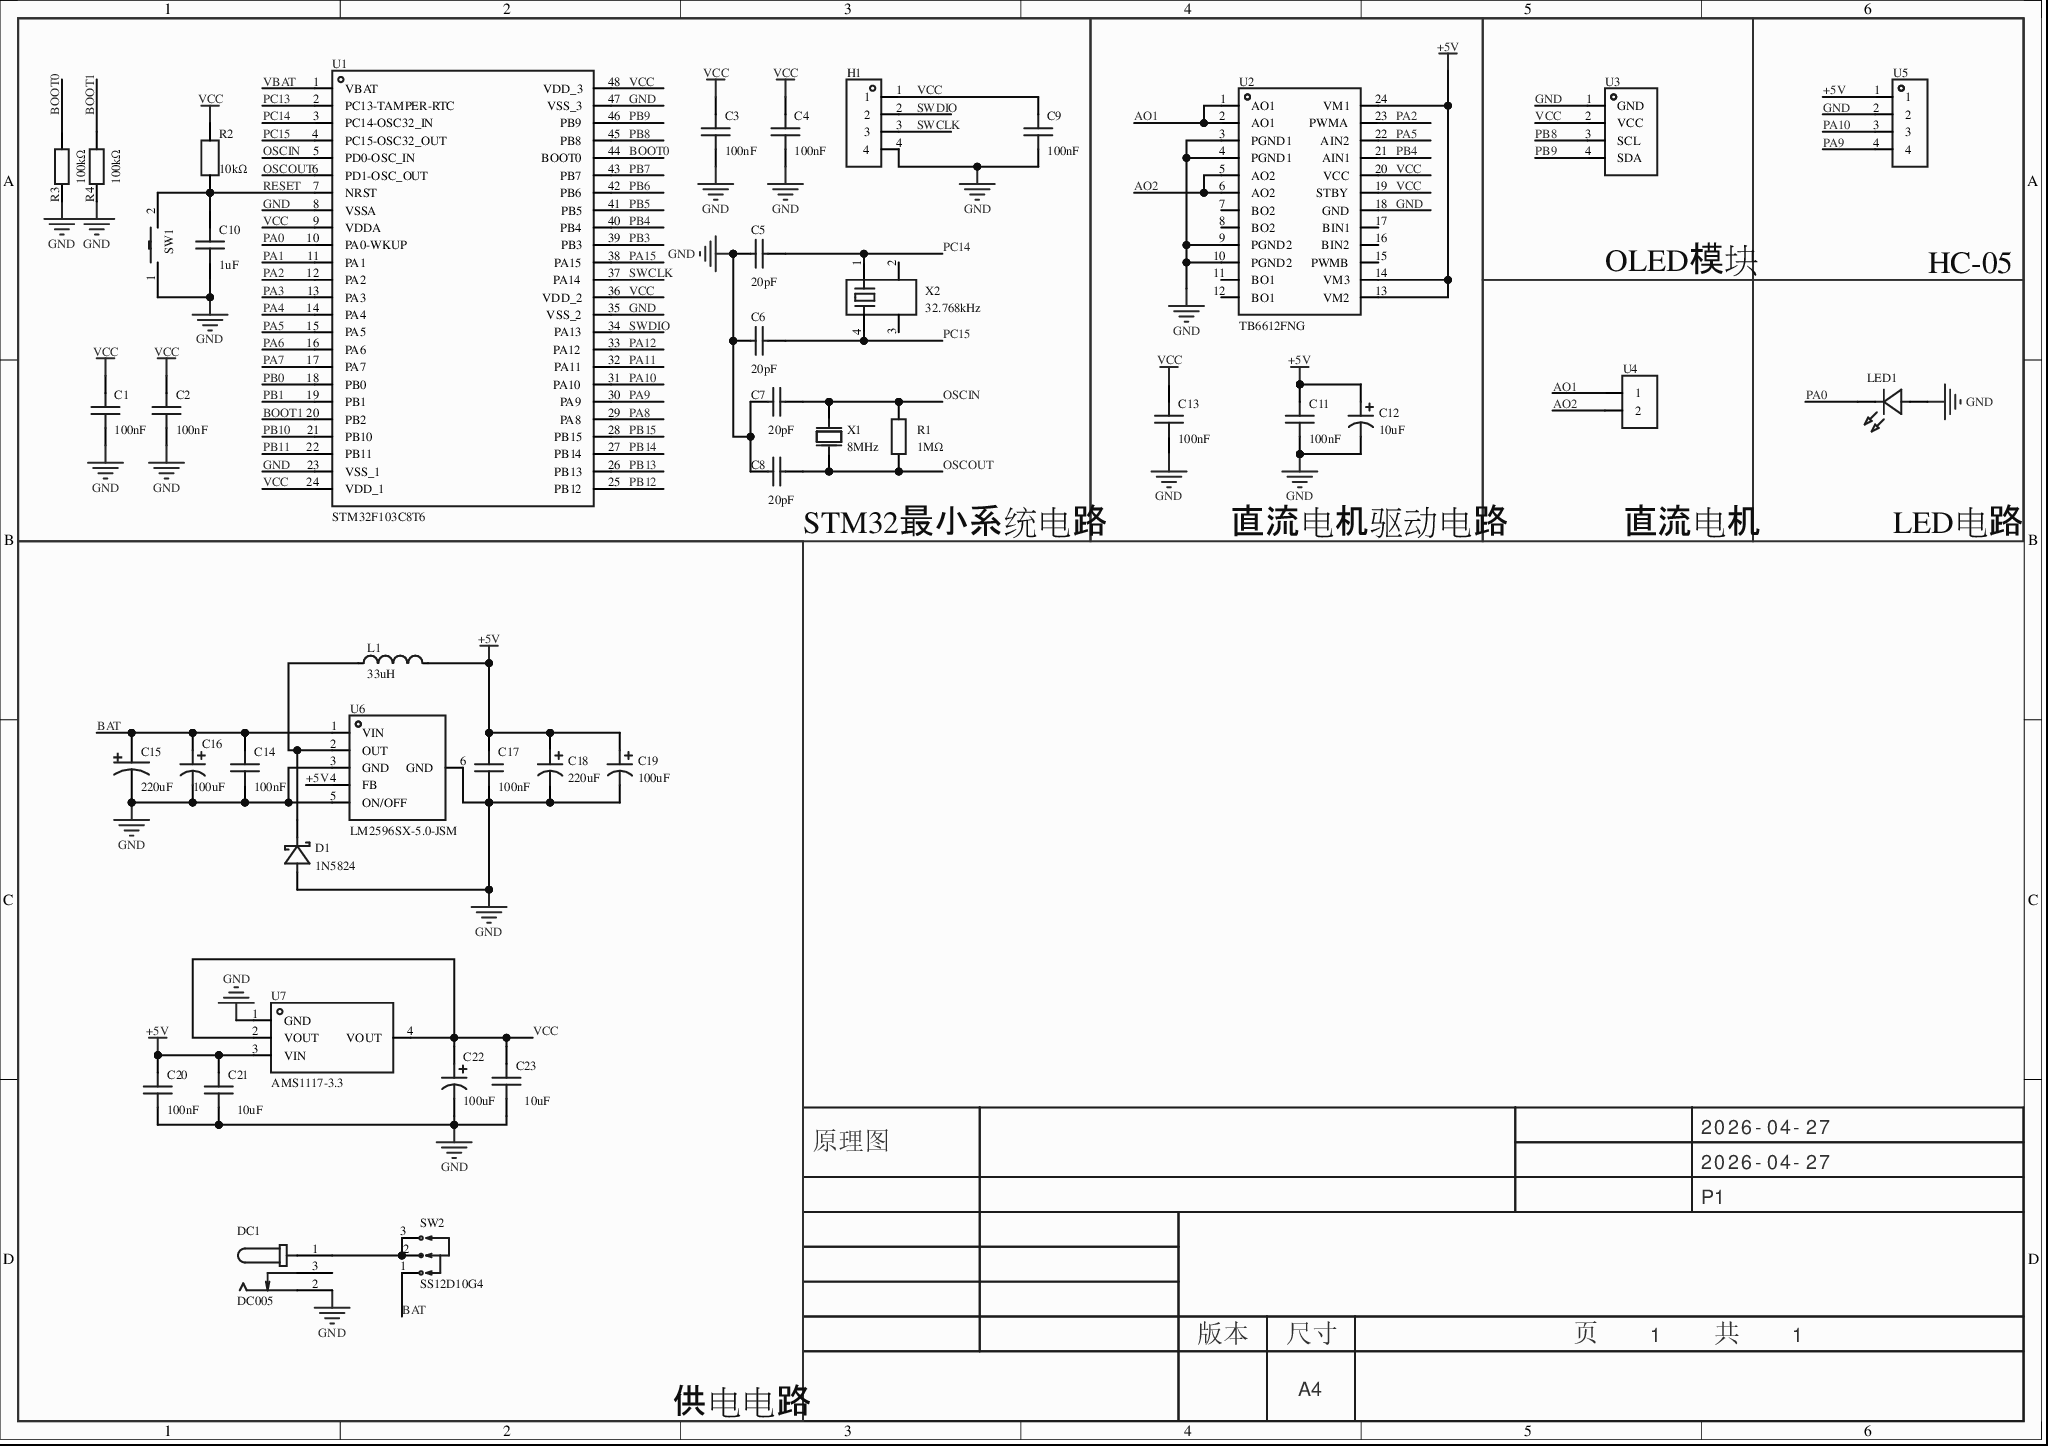
[diagram p0: MISC51997-3.schdoc]
# Altium project MISC51997-2.PrjPcb
1 sheet, 43 parts. Net scope: global (net labels, ports and power ports of the same name join across sheets).
Board file: MISC51997.pcbdoc

## Sheet MISC51997-3.schdoc
size 297 x 209 mm; Version: V1.0; @Project Name: MISC51997; @Update Date: 2026-04-27; @Create Date: 2026-04-27; @Board Name: MISC51997; @Create Time: 21:08:27; @Page Count: 1; @Page No: 1; @Schematic Name: MISC51997; @Update Time: 21:08:27; Size: A4

### Parts
C1  100nF  [C0603]
C2  100nF  [C0603]
C3  100nF  [C0603]
C4  100nF  [C0603]
C5  20pF  [C0603]
C6  20pF  [C0603]
C7  20pF  [C0603]
C8  20pF  [C0603]
C9  100nF  [C0603]
C10  1uF  [C0603]
C11  100nF  [C0603]
C12  10uF  [CAP-TH_BD5.0-P2.00-D0.5-FD-A]
C13  100nF  [C0603]
C14  100nF  [C0603]
C15  220uF  [CAP-TH_BD10.0-P5.00-D1.0-FD]
C16  100uF  [CAP-TH_BD6.3-P2.50-D0.5-FD]
C17  100nF  [C0603]
C18  220uF  [CAP-TH_BD6.3-P2.50-D0.5-FD_DXW025M227E112S1AA]
C19  100uF  [CAP-TH_BD6.3-P2.50-D0.5-FD]
C20  100nF  [C0603]
C21  10uF  [C0805]
C22  100uF  [CAP-TH_BD6.3-P2.50-D0.5-FD]
C23  10uF  [C0805]
D1  1N5824  [DO-201AD_BD5.3-L9.0-P13.00-D1.3-RD]
DC1  DC005  [DC-IN-TH_DC005]
H1  PZ254R-11-04P  [HDR-TH_4P-P2.54-H-M-W10.4]  (value not drawn)
L1  33uH  [IND-SMD_L3.5-W3.0]
LED1  BL-BUB1V4V-AT  [LED-TH_BD5.8-P2.54-FD_RED]  (value not drawn)
R1  1MΩ  [R0603]
R2  10kΩ  [R0603]
R3  100kΩ  [R0603]
R4  100kΩ  [R0603]
SW1  TS-1101-C-W  [SW-SMD_L6.0-W3.3-LS8.0_TS-1101-C-W]  (value not drawn)
SW2  SS12D10G4  [SW-TH_3P-P4.80-HX-SS12D10G4]
U1  STM32F103C8T6  [LQFP-48_L7.0-W7.0-P0.50-LS9.0-BL]
U2  TB6612FNG  [SSOP-24_L8.4-W5.8-P0.65-LS7.8-BL]
U3  HS96L03W2C03  [OLED-TH_L27.8-W27.2-P2.54_C9900033791]  (value not drawn)
U4  2.54-1*2P母  [HDR-TH_2P-P2.54-V-F]  (value not drawn)
U5  2.54-1*4P母  [HDR-TH_4P-P2.54-V-F]  (value not drawn)
U6  LM2596SX-5.0-JSM  [TO-263-5_L10.0-W8.4-P1.70-LS15.3-BR]
U7  AMS1117-3.3  [SOT-223-3_L6.5-W3.4-P2.30-LS7.0-BR]
X1  8MHz  [OSC-TH_L10.0-W4.5-P5.00]
X2  32.768kHz  [MC-306_4P-L8.0-W3.2-P5.5-BL]

### Blocks framed on the sheet
STM32最小系统电路: C1-C10 H1 R1-R4 SW1 U1 X1 X2
直流电机驱动电路: C11-C13 U2
OLED模块: U3
HC-05: U5
供电电路: C14-C23 D1 DC1 L1 SW2 U6 U7

### Nets
+5V: C11.2 C12.1 C17.2 C18.1 C19.1 C20.2 C21.2 L1.2 U2.13(VM2) U2.14(VM3) U2.24(VM1) U5.1 U6.4(FB) U7.3(VIN)
GND: C1.1 C2.1 C3.1 C4.1 C5.2 C6.2 C7.2 C8.2 C9.1 C10.1 C11.1 C12.2 C13.1 C14.1 C15.2 C16.2 C17.1 C18.2 C19.2 C20.1 C21.1 C22.2 C23.1 D1.2(A) DC1.2 H1.4 LED1.1(A) R3.1 R4.1 SW1.1 U1.8(VSSA) U1.23(VSS_1) U1.35(VSS_2) U1.47(VSS_3) U2.3(PGND1) U2.4(PGND1) U2.9(PGND2) U2.10(PGND2) U2.18(GND) U3.1(GND) U5.2 U6.3(GND) U6.5(ON/OFF) U6.6(GND) U7.1(GND)
VCC: C1.2 C2.2 C3.2 C4.2 C9.2 C13.2 C22.1 C23.2 H1.1 R2.2 U1.9(VDDA) U1.24(VDD_1) U1.36(VDD_2) U1.48(VDD_3) U2.19(STBY) U2.20(VCC) U3.2(VCC) U7.2(VOUT) U7.4(VOUT)
AO1: U2.1(AO1) U2.2(AO1) U4.1
AO2: U2.5(AO2) U2.6(AO2) U4.2
BAT: C14.2 C15.1 C16.1 SW2.1 U6.1(VIN)
BOOT0: R3.2 U1.44(BOOT0)
BOOT1: R4.2 U1.20(PB2)
OSCIN: C7.1 R1.2 U1.5(PD0-OSC_IN) X1.1(OSC1)
OSCOUT: C8.1 R1.1 U1.6(PD1-OSC_OUT) X1.2(OSC2)
PA0: LED1.2(K) U1.10(PA0-WKUP)
PA1: U1.11(PA1)
PA2: U1.12(PA2) U2.23(PWMA)
PA3: U1.13(PA3)
PA4: U1.14(PA4)
PA5: U1.15(PA5) U2.22(AIN2)
PA6: U1.16(PA6)
PA7: U1.17(PA7)
PA8: U1.29(PA8)
PA9: U1.30(PA9) U5.4
PA10: U1.31(PA10) U5.3
PA11: U1.32(PA11)
PA12: U1.33(PA12)
PA15: U1.38(PA15)
PB0: U1.18(PB0)
PB1: U1.19(PB1)
PB3: U1.39(PB3)
PB4: U1.40(PB4) U2.21(AIN1)
PB5: U1.41(PB5)
PB6: U1.42(PB6)
PB7: U1.43(PB7)
PB8: U1.45(PB8) U3.3(SCL)
PB9: U1.46(PB9) U3.4(SDA)
PB10: U1.21(PB10)
PB11: U1.22(PB11)
PB12: U1.25(PB12)
PB13: U1.26(PB13)
PB14: U1.27(PB14)
PB15: U1.28(PB15)
PC13: U1.2(PC13-TAMPER-RTC)
PC14: C5.1 U1.3(PC14-OSC32_IN) X2.1
PC15: C6.1 U1.4(PC15-OSC32_OUT) X2.4
RESET: C10.2 R2.1 SW1.2 U1.7(NRST)
SWCLK: H1.3 U1.37(PA14)
SWDIO: H1.2 U1.34(PA13)
VBAT: U1.1(VBAT)
NetD1_1: D1.1(K) L1.1 U6.2(OUT)
NetDC1_1: DC1.1 SW2.2 SW2.3

Not connected (* = marked no-connect by the designer): DC1 3; U2 7(BO2)* 8(BO2)* 11(BO1)* 12(BO1)* 15(PWMB)* 16(BIN2)* 17(BIN1)*; X2 2 3

### Notes on the sheet
- 直流电机
- LED电路
- 2026-04-27
- 原理图
- P1
- 版本
- 尺寸
- A4
- 页    1    共    1

### Library data of the parts
C1-C4 C9 C11 C13 C14 C17 C20 = CGA0603X7R104K500JT: 容值:100nF;精度:±10%;额定电压:50V;温度系数:X7R;; Manufacturer: HRE(芯声); 3D Model: ac125912035d415993ca9572d50418b10819f05c4eef4c71ace90d822a990e87; 3D Model Transform: 62.992,31.496,0,0,0,0,0,0,0; Tolerance: ±10%; Voltage Rating: 50V; Temperature Coefficient: X7R; AddInBom: yes; ModelName: C0603_L1.6-W0.8-H0.8; Symbol: CGA0603X7R104K500JT; Device: CGA0603X7R104K500JT; LCSC Part Name: 100nF ±10% 50V; Supplier Part: C6119867; Manufacturer Part: CGA0603X7R104K500JT; Supplier Footprint: 0603; JLCPCB Part Class: Extended Part; Datasheet: https://item.szlcsc.com/datasheet/CGA0603X7R104K500JT/7062573.html; Supplier: LCSC; Value: 100nF; ConvertToPcb: yes; FootprintName: C0603
C5-C8 = CL10C200JB8NNNC: 容值:20pF;精度:±5%;额定电压:50V;温度系数:C0G;; Manufacturer: SAMSUNG(三星); 3D Model: ac125912035d415993ca9572d50418b10819f05c4eef4c71ace90d822a990e87; 3D Model Transform: 62.992,31.496,0,0,0,0,0,0,0; Tolerance: ±5%; Voltage Rating: 50V; Temperature Coefficient: C0G; AddInBom: yes; ModelName: C0603_L1.6-W0.8-H0.8; Symbol: CL10C200JB8NNNC; Device: CL10C200JB8NNNC; LCSC Part Name: 20pF ±5% 50V; Supplier Part: C1648; Manufacturer Part: CL10C200JB8NNNC; Supplier Footprint: 0603; JLCPCB Part Class: Basic Part; Datasheet: https://item.szlcsc.com/datasheet/CL10C200JB8NNNC/2000.html; Supplier: LCSC; Value: 20pF; ConvertToPcb: yes; FootprintName: C0603
C10 = CC0603KRX7R9BB105: 容值:1uF;精度:±10%;额定电压:50V;温度系数:X7R;; Manufacturer: YAGEO(国巨); 3D Model: ac125912035d415993ca9572d50418b10819f05c4eef4c71ace90d822a990e87; 3D Model Transform: 62.992,31.496,0,0,0,0,0,0,0; Tolerance: ±10%; Voltage Rating: 50V; Temperature Coefficient: X7R; AddInBom: yes; ModelName: C0603_L1.6-W0.8-H0.8; Symbol: CC0603KRX7R9BB105; Device: CC0603KRX7R9BB105; LCSC Part Name: 1uF ±10% 50V; Supplier Part: C559769; Manufacturer Part: CC0603KRX7R9BB105; Supplier Footprint: 0603; JLCPCB Part Class: Extended Part; Datasheet: https://item.szlcsc.com/datasheet/CC0603KRX7R9BB105/584032.html; Supplier: LCSC; Value: 1uF; ConvertToPcb: yes; FootprintName: C0603
C12 = ERG50V10M5X11: 容值:10uF;精度:±20%;额定电压:50V;纹波电流:180mA@100kHz;等效串联电阻(ESR):1.3Ω@100kHz;; Manufacturer: JIERR(捷而瑞); 3D Model: 230b3bd6484f4b52b9cf74c8bd6c61990819f05c4eef4c71ace90d822a990e87; 3D Model Transform: 197.2437,197.23953,0,0,0,0,0,0,-196.85; Tolerance: ±20%; Voltage Rating: 50V; Pin Spacing: 2mm; Lifetime: 2000hrs@105℃; AddInBom: yes; Symbol: ERG50V10M5X11; Device: ERG50V10M5X11; LCSC Part Name: 10uF ±20% 50V; Supplier Part: C47344184; Manufacturer Part: ERG50V10M5X11; Supplier Footprint: 插件,D5xL11mm; JLCPCB Part Class: Extended Part; Datasheet: https://item.szlcsc.com/datasheet/ERG50V10M5X11/49556625.html; Supplier: LCSC; Value: 10uF; Ripple Current: 180mA@100kHz; Equivalent Series Resistance(ESR): 1.3Ω@100kHz; Diameter: 5mm; Height - Seated (Max): 11mm; Operating Temperature: -40℃~+105℃; ConvertToPcb: yes; FootprintName: CAP-TH_BD5.0-P2.00-D0.5-FD-A; ModelName: CAP-TH_BD5.0-P2.00-D0.5-FD-A
C15 = ECRE1013221M050P00: 容值:220uF;精度:±20%;额定电压:50V;纹波电流:-;等效串联电阻(ESR):-;; Manufacturer: TOPAZ(黄宝石); 3D Model: 6ce78ce5315348e095d700085da75e480819f05c4eef4c71ace90d822a990e87; 3D Model Transform: 394.094,393.72252,0,0,0,0,0,0,-137.795; Tolerance: ±20%; Voltage Rating: 50V; Pin Spacing: 5mm; Lifetime: 2000hrs@105℃; AddInBom: yes; ModelName: CAP-TH_D10.0-H16.0-P5.00; Symbol: ECRE1013221M050P00; Device: ECRE1013221M050P00; LCSC Part Name: 220uF ±20% 50V; Supplier Part: C156787; Manufacturer Part: ECRE1013221M050P00; Supplier Footprint: 插件,D10xL13mm; JLCPCB Part Class: Extended Part; Datasheet: https://item.szlcsc.com/datasheet/ECRE1013221M050P00/168132.html; Supplier: LCSC; Value: 220uF; Ripple Current: -; Equivalent Series Resistance(ESR): -; Diameter: 10mm; Height - Seated (Max): 13mm; ConvertToPcb: yes; FootprintName: CAP-TH_BD10.0-P5.00-D1.0-FD
C16 = DXW050M107E122S1AA: 容值:100uF;精度:±20%;额定电压:50V;纹波电流:555mA@100KHz;; Manufacturer: KNSCHA(科尼盛); 3D Model: 983aa343eddc42b59ebb10541a88166e0819f05c4eef4c71ace90d822a990e87; 3D Model Transform: 247.99486,248.229,0,90,0,0,0,0,-196.85; Tolerance: ±20%; Voltage Rating: 50V; Lifetime: 5000hrs@105℃; AddInBom: yes; Symbol: DXW050M107E122S1AA; Device: DXW050M107E122S1AA; LCSC Part Name: 100UF ±20% 50V; Supplier Part: C42416626; Manufacturer Part: DXW050M107E122S1AA; Supplier Footprint: 插件,D6.3xL12mm; JLCPCB Part Class: Extended Part; Datasheet: https://item.szlcsc.com/datasheet/DXW050M107E122S1AA/44417370.html; Supplier: LCSC; Value: 100uF; Ripple Current: 555mA@100KHz; Operating Temperature: -40℃~+105℃; ConvertToPcb: yes; FootprintName: CAP-TH_BD6.3-P2.50-D0.5-FD; ModelName: CAP-TH_BD6.3-P2.50-D0.5-FD
C18 = DXW025M227E112S1AA: 容值:220uF;精度:±20%;额定电压:25V;纹波电流:640mA@100KHz;; Manufacturer: KNSCHA(科尼盛); Tolerance: ±20%; Voltage Rating: 25V; Lifetime: 5000hrs@105℃; AddInBom: yes; Symbol: DXW025M227E112S1AA; Device: DXW025M227E112S1AA; LCSC Part Name: 220UF ±20% 25V; Supplier Part: C42416623; Manufacturer Part: DXW025M227E112S1AA; Supplier Footprint: 插件,D6.3xL11mm; Datasheet: https://item.szlcsc.com/datasheet/DXW025M227E112S1AA/44417367.html; Supplier: LCSC; Value: 220uF; Ripple Current: 640mA@100KHz; Operating Temperature: -40℃~+105℃; ConvertToPcb: yes; FootprintName: CAP-TH_BD6.3-P2.50-D0.5-FD_DXW025M227E112S1AA
C19 C22 = 100uF16V6.3x11KM: 容值:100uF;精度:±20%;额定电压:16V;纹波电流:142mA@120Hz;; Manufacturer: Econd(米朗电子); 3D Model: 983aa343eddc42b59ebb10541a88166e0819f05c4eef4c71ace90d822a990e87; 3D Model Transform: 247.99486,248.229,0,90,0,0,0,0,-196.85; Tolerance: ±20%; Voltage Rating: 16V; Pin Spacing: 2.5mm; Lifetime: 2000hrs@105℃; AddInBom: yes; Symbol: 100UF16V6.3X11KM; Device: 100uF16V6.3x11KM; LCSC Part Name: 100uF ±20% 16V; Supplier Part: C49304900; Manufacturer Part: 100uF16V6.3x11KM; Supplier Footprint: 插件,D6.3xL11mm; JLCPCB Part Class: Extended Part; Datasheet: https://item.szlcsc.com/datasheet/100uF16V6.3x11KM/51766728.html; Supplier: LCSC; Value: 100uF; Ripple Current: 142mA@120Hz; Diameter: 6.3mm; Height - Seated (Max): 11mm; Operating Temperature: -40℃~+105℃; ConvertToPcb: yes; FootprintName: CAP-TH_BD6.3-P2.50-D0.5-FD; ModelName: CAP-TH_BD6.3-P2.50-D0.5-FD
C21 C23 = CGA0805X5R106K250MT: 容值:10uF;精度:±10%;额定电压:25V;温度系数:X5R;; Manufacturer: HRE(芯声); 3D Model: 1ba041120af144c991958decab20d2410819f05c4eef4c71ace90d822a990e87; 3D Model Transform: 78.74,51.181,0,0,0,0,0,0.0005,0; Tolerance: ±10%; Voltage Rating: 25V; Temperature Coefficient: X5R; AddInBom: yes; ModelName: C0805_L2.0-W1.3-H1.3; Symbol: CGA0805X5R106K250MT; Device: CGA0805X5R106K250MT; LCSC Part Name: 10uF ±10% 25V; Supplier Part: C6119887; Manufacturer Part: CGA0805X5R106K250MT; Supplier Footprint: 0805; JLCPCB Part Class: Extended Part; Datasheet: https://item.szlcsc.com/datasheet/CGA0805X5R106K250MT/7062593.html; Supplier: LCSC; Value: 10uF; ConvertToPcb: yes; FootprintName: C0805
D1 = 1N5824_C27636124: Manufacturer: DOWO(东沃); 3D Model: 03764715b90b46d9aad58598935395240819f05c4eef4c71ace90d822a990e87; 3D Model Transform: 562.991,209.02013,0,0,0,0,0,0,-196.85; AddInBom: yes; Symbol: 1N5824_C27636124; Device: 1N5824_C27636124; LCSC Part Name: 1N5824; Supplier Part: C27636124; Manufacturer Part: 1N5824; Supplier Footprint: DO-201AD; JLCPCB Part Class: Extended Part; Datasheet: https://item.szlcsc.com/datasheet/1N5824/29373159.html; Supplier: LCSC; ConvertToPcb: yes; FootprintName: DO-201AD_BD5.3-L9.0-P13.00-D1.3-RD; ModelName: DO-201AD_BD5.3-L9.0-P13.00-D1.3-RD
DC1 = DC005: 连接器类型:DC电源插座;安装方式:弯插;触点内径:2mm;触点外径:6.3mm;额定电流:500mA;额定电压:12V;工作温度:-30℃~+70℃;; Manufacturer: SHOU HAN(首韩); Symbol: DC005_C431533; 3D Model: f168fe383f964e0ea2af0127ff6ac7b40819f05c4eef4c71ace90d822a990e87; 3D Model Transform: 366.141,553.149,0,270,0,0,-141.734,88.583,-149.606; Connector Type: DC电源插座; Inside Contact Diameter: 2mm; Outside Contact Diameter: 6.3mm; Current Rating: 500mA; Voltage Rating (Max): 12V; AddInBom: yes; Device: DC005; LCSC Part Name: DC005-2.0 黑（铁）; Supplier Part: C431533; Manufacturer Part: DC005; Supplier Footprint: 插件; JLCPCB Part Class: Extended Part; Datasheet: https://item.szlcsc.com/datasheet/DC005/427890.html; Supplier: LCSC; Mounting Type: 弯插; Operating Temperature: -30℃~+70℃; ConvertToPcb: yes; FootprintName: DC-IN-TH_DC005; ModelName: DC-IN-TH_DC005
H1 = PZ254R-11-04P: 插针结构:1x4P;间距:2.54mm;行距:-;圆针/方针:方针;安装方式:弯插;排数:单排;总PIN位数:4P;额定电流:3A;额定电压:250V;配合针长度:6mm;塑高:2.5mm;端接针长度:-;触头材质:黄铜;触头镀层:-;工作温度:-40℃~+105℃;颜色:黑色;; Manufacturer: XFCN(兴飞); 3D Model: d6c429cf28314298a2074cefd68172f00819f05c4eef4c71ace90d822a990e87; 3D Model Transform: 399.999,417.322,0,180,0,0,0,-196.85,-118.11; Pin Structure: 1x4P; Pitch: 2.54mm; Circluar Pins/Square Pins: 方针; Current Rating: 3A; Voltage Rating (Max): 250V; AddInBom: yes; ModelName: HDR-TH_4P-P2.54-M-WI-1X4P; Symbol: PZ254R-11-04P; Device: PZ254R-11-04P; LCSC Part Name: 1x4P 间距:2.54mm 方针 弯插; Supplier Part: C492412; Manufacturer Part: PZ254R-11-04P; Supplier Footprint: 弯插,P=2.54mm; JLCPCB Part Class: Extended Part; Datasheet: https://item.szlcsc.com/datasheet/PZ254R-11-04P/502968.html; Supplier: LCSC; Row Spacing: -; Mounting Type: 弯插; Number of Rows: 单排; Number of Pins: 4P; Length of Mating Pin: 6mm; Insulation Height: 2.5mm; Length of End Connection Pin: -; Contact Material: 黄铜; Contact Plating: -; Operating Temperature: -40℃~+105℃; Color: 黑色; ConvertToPcb: yes; FootprintName: HDR-TH_4P-P2.54-H-M-W10.4
L1 = YP0301-330M: 电感值:33uH;精度:±20%;额定电流:240mA;; Manufacturer: YJYCOIN(益嘉源); 3D Model: 7453ea2b43e849b9af19fd0bdb505bea0819f05c4eef4c71ace90d822a990e87; 3D Model Transform: 118.11,131.556,0,90,0,0,0,0,0; Tolerance: ±20%; Current Rating: 240mA; DC Resistance(DCR): 2.888Ω; AddInBom: yes; ModelName: IND-SMD_L3.5-W3.0-H2.0; Symbol: YP0301-330M; Device: YP0301-330M; LCSC Part Name: 33uH ±20%; Supplier Part: C576562; Manufacturer Part: YP0301-330M; Supplier Footprint: SMD,3.5x3mm; JLCPCB Part Class: Extended Part; Datasheet: https://item.szlcsc.com/datasheet/YP0301-330M/604053.html; Supplier: LCSC; Value: 33uH; ConvertToPcb: yes; FootprintName: IND-SMD_L3.5-W3.0
LED1 = BL-BUB1V4V-AT: 发光颜色:红色;正向电流:-;; Manufacturer: BrtLed(佰鸿); 3D Model: cd10af5921d54ca5b2eb89b15bce9caa0819f05c4eef4c71ace90d822a990e87; 3D Model Transform: 212.63737,227.928,0,0,0,0,-7.874,0,-196.85; Illumination Color: 红色; AddInBom: yes; Symbol: BL-BUB1V4V; Device: BL-BUB1V4V-AT; LCSC Part Name: F4.98红发红红光; Supplier Part: C7421379; Manufacturer Part: BL-BUB1V4V-AT; Supplier Footprint: 插件; JLCPCB Part Class: Extended Part; Datasheet: https://item.szlcsc.com/datasheet/BL-BUB1V4V-AT/8401795.html; Supplier: LCSC; Forward Current: -; ConvertToPcb: yes; FootprintName: LED-TH_BD5.8-P2.54-FD_RED; ModelName: LED-TH_BD5.8-P2.54-FD_RED
R1 = 0603WAF1004T5E: 电阻类型:厚膜电阻;阻值:1MΩ;精度:±1%;功率:100mW;最大工作电压:75V;温度系数:±100ppm/℃;; Manufacturer: UNI-ROYAL(厚声); 3D Model: fc143cca1e79419f9cd78b61e9279f080819f05c4eef4c71ace90d822a990e87; 3D Model Transform: 31.8897,63.7794,0,90,0,0,0,0,0; Tolerance: ±1%; Power(Watts): 100mW; Overload Voltage (Max): 75V; AddInBom: yes; Symbol: 0603WAF1004T5E; Device: 0603WAF1004T5E; LCSC Part Name: 1MΩ ±1% 100mW 厚膜电阻; Supplier Part: C22935; Manufacturer Part: 0603WAF1004T5E; Supplier Footprint: 0603; JLCPCB Part Class: Basic Part; Datasheet: https://atta.szlcsc.com/upload/public/pdf/source/20200306/C422600_1E6D84923E4A46A82E41ADD87F860B5C.pdf; Supplier: LCSC; Type: 厚膜电阻; Value: 1MΩ; Temperature Coefficient: ±100ppm/℃; Operating Temperature Range: -55℃~+155℃; ConvertToPcb: yes; FootprintName: R0603; ModelName: R0603
R2 = FRC0603F1002TS: 电阻类型:厚膜电阻;阻值:10kΩ;精度:±1%;功率:100mW;工作电压:75V;温度系数:±100ppm/℃;; Manufacturer: FOJAN(富捷); 3D Model: fc143cca1e79419f9cd78b61e9279f080819f05c4eef4c71ace90d822a990e87; 3D Model Transform: 31.8897,63.7794,0,90,0,0,0,0,0; Tolerance: ±1%; Power(Watts): 100mW; Voltage-Supply(Max): 75V; AddInBom: yes; Symbol: FRC0603F1002TS; Device: FRC0603F1002TS; LCSC Part Name: 10kΩ ±1% 100mW 厚膜电阻; Supplier Part: C2906982; Manufacturer Part: FRC0603F1002TS; Supplier Footprint: 0603; JLCPCB Part Class: Extended Part; Supplier: LCSC; Type: 厚膜电阻; Value: 10kΩ; Temperature Coefficient: ±100ppm/℃; Operating Temperature: -55℃~+155℃; ConvertToPcb: yes; FootprintName: R0603; ModelName: R0603
R3 R4 = 0603WAF1003T5E: 电阻类型:厚膜电阻;阻值:100kΩ;精度:±1%;功率:100mW;工作电压:75V;温度系数:±100ppm/℃;; Manufacturer: UNI-ROYAL(厚声); 3D Model: fc143cca1e79419f9cd78b61e9279f080819f05c4eef4c71ace90d822a990e87; 3D Model Transform: 31.8897,63.7794,0,90,0,0,0,0,0; Tolerance: ±1%; Power(Watts): 100mW; Voltage-Supply(Max): 75V; AddInBom: yes; Symbol: 0603WAF1003T5E; Device: 0603WAF1003T5E; LCSC Part Name: 100kΩ ±1% 100mW 厚膜电阻; Supplier Part: C25803; Manufacturer Part: 0603WAF1003T5E; Supplier Footprint: 0603; JLCPCB Part Class: Basic Part; Datasheet: https://item.szlcsc.com/datasheet/0603WAF1003T5E/26546.html; Supplier: LCSC; Type: 厚膜电阻; Value: 100kΩ; Temperature Coefficient: ±100ppm/℃; Operating Temperature: -55℃~+155℃; ConvertToPcb: yes; FootprintName: R0603; ModelName: R0603
SW1 = TS-1101-C-W: 电路结构:单刀单掷;按钮形状:矩形按钮;作用力:2.6N;安装方式:立贴;开关长度:6mm;开关宽度:3.6mm;开关高度:2.5mm;带支架:不带支架;触点电流:50mA;额定电压:12V;带灯:无;工作寿命:5万次;; Manufacturer: XKB Connection(中国星坤); 3D Model: 0fd6340cfb7d45bfbbb5f8576d023f850819f05c4eef4c71ace90d822a990e87; 3D Model Transform: 315.232,145.669,0,0,0,0,0,0,0; Circuit: 单刀单掷; Actuator Style: 矩形按钮; Operating Force: 2.6N; Switch Height: 2.5mm; with Bracket: 不带支架; Contact Current: 50mA; Voltage Rating: 12V; With Lamp: 无; Life: 5万次; AddInBom: yes; Symbol: TS-1101-C-W; Device: TS-1101-C-W; LCSC Part Name: 6*3.6*2.5mm 立贴 轻触开关; Supplier Part: C318938; Manufacturer Part: TS-1101-C-W; Supplier Footprint: SMD,6x3.6mm; JLCPCB Part Class: Extended Part; Datasheet: https://item.szlcsc.com/datasheet/TS-1101-C-W/300030.html; Supplier: LCSC; Mounting Type: 立贴; Length: 6mm; Width: 3.6mm; Actuator/Cap Color: -; IP Rating: -; Termination Style: -; Operating Temperature: -30℃~+85℃; ConvertToPcb: yes; FootprintName: SW-SMD_L6.0-W3.3-LS8.0_TS-1101-C-W; ModelName: SW-SMD_L6.0-W3.3-LS8.0_TS-1101-C-W
SW2 = SS12D10G4: 电路结构:单刀双掷;安装方式:直插;开关颜色:黑色;额定电流:2A;额定电压:125V;; Manufacturer: HanElectricity(瀚源); 3D Model: cfce8581009a45839cc96a3fa85751f80819f05c4eef4c71ace90d822a990e87; 3D Model Transform: 499.999,263.779,0,0,0,0,-0.589,-0.591,-196.85; Circuit: 单刀双掷; Actuator Style: 矩形柱状; Actuator Color: 黑色; Current Rating: 2A; Voltage Rating: 125V; AddInBom: yes; ModelName: SW-TH_SHOU-HAN_SS12D10G4; Symbol: SS12D10G4; Device: SS12D10G4; LCSC Part Name: SS12D10G4; Supplier Part: C48601060; Manufacturer Part: SS12D10G4; Supplier Footprint: 插件; JLCPCB Part Class: Extended Part; Datasheet: https://item.szlcsc.com/datasheet/SS12D10G4/50871456.html; Supplier: LCSC; Termination Style: PC引脚; Length: 12.7mm; Width: 6.7mm; Mounting Type: 直插; Operating Temperature: -16℃~+60℃; ConvertToPcb: yes; FootprintName: SW-TH_3P-P4.80-HX-SS12D10G4
U1 = STM32F103C8T6: CPU内核:ARM-M3;CPU最大主频:72MHz;应用领域:-;; Manufacturer: ST(意法半导体); 3D Model: 093be70396ff421eb2cdb946d5311efc0819f05c4eef4c71ace90d822a990e87; 3D Model Transform: 354.331,354.331,0,0,0,0,0,0,0; CPU Core: ARM-M3; CPU Maximum Speed: 72MHz; Program Storage Size: 64KB; Program Memory Type: FLASH; Number of I/O: 37; ADC (Bit): 12bit; Voltage - Supply: 2V~3.6V; AddInBom: yes; ModelName: LQFP-48_L7.0-W7.0-H1.4-LS9.0-P0.50; Symbol: STM32F103C8T6; Device: STM32F103C8T6; LCSC Part Name: 主流增强型ARM Cortex-M3 MCU，具有64 KB Flash、72 MHz CPU、电机控制、USB和CAN; Supplier Part: C8734; Manufacturer Part: STM32F103C8T6; Supplier Footprint: LQFP-48(7x7); JLCPCB Part Class: Extended Part; Datasheet: https://item.szlcsc.com/datasheet/STM32F103C8T6/9243.html; Supplier: LCSC; Applications: -; ConvertToPcb: yes; FootprintName: LQFP-48_L7.0-W7.0-P0.50-LS9.0-BL
U2 = TB6612FNG(O,C,8,EL: 双直流电机驱动器集成电路; Manufacturer: TOSHIBA(东芝); 3D Model: 66f9840b265a41cbab4a1bbd068cd8690819f05c4eef4c71ace90d822a990e87; 3D Model Transform: 303.12939,330.708,0,90,0,0,0,-0.0005,0; Number of H-bridges: 2; Output Current: 1A; Peak Current: 3.2A; Voltage - Supply: 2.7V~5.5V; RDS(on): 500mΩ; Quiescent Current(Iq): 1uA; AddInBom: yes; ModelName: SSOP-24_L8.4-W5.3-H2.0-LS7.8-P0.65; Symbol: TB6612FNG(O,C,8,EL; Device: TB6612FNG(O,C,8,EL; LCSC Part Name: 双直流电机驱动IC; Supplier Part: C88224; Manufacturer Part: TB6612FNG; Supplier Footprint: SSOP-24-208mil; JLCPCB Part Class: Extended Part; Datasheet: https://item.szlcsc.com/datasheet/TB6612FNG(O%252CC%252C8%252CEL/89402.html; Supplier: LCSC; Technology: 是; Operating Temperature: -20℃~+85℃; ConvertToPcb: yes; FootprintName: SSOP-24_L8.4-W5.8-P0.65-LS7.8-BL
U3 = HS96L03W2C03: 核心芯片:SSD1315芯片;接口类型:I2C;尺寸(inch):0.96;像素分辨率:128x64;; Manufacturer: HS(汉昇); 3D Model: bb65183306db4ca69fb52250be49b00e0819f05c4eef4c71ace90d822a990e87; 3D Model Transform: 1070.864,1094.486,0,0,0,0,0,-498.424,0; Interface: I2C; Dot Pixels: 128x64; Type of Drive: 无源(PMOLED); Display Range: 21.744x10.864mm; Display Color: 白色; Luminance: 180cd/m2; AddInBom: yes; Symbol: HS96L03W2C03; Device: HS96L03W2C03; LCSC Part Name: 0.96寸OLED显示屏窄白光IIC; Supplier Part: C5248080; Manufacturer Part: HS96L03W2C03; Supplier Footprint: -; JLCPCB Part Class: Extended Part; Datasheet: https://item.szlcsc.com/datasheet/HS96L03W2C03/5960631.html; Supplier: LCSC; Controller Type: SSD1315芯片; Size: 0.96; Operating Temperature: -40℃~+70℃; Function: -; Quiescent Current: -; ConvertToPcb: yes; FootprintName: OLED-TH_L27.8-W27.2-P2.54_C9900033791; ModelName: OLED-TH_L27.8-W27.2-P2.54_C9900033791
U4 = 2.54-1*2P母: 插孔结构:1x2P;间距:2.54mm;行距:-;圆孔/方孔:方孔;安装方式:直插;排数:单排;总孔位数:2P;额定电流:3A;额定电压:-;插孔方向:顶部;塑高:-;触头材质:黄铜;触头镀层:-;工作温度:-40℃~+105℃;; Manufacturer: BOOMELE(博穆精密); Symbol: Header-Female-2.54_1x2; 3D Model: a9450ef445564560a104363b9aacde4e0819f05c4eef4c71ace90d822a990e87; 3D Model Transform: 215.7476,98.425,0,0,0,0,0,0,-129.921; Holes Structure: 1x2P; Pitch: 2.54mm; Circular Hole / Square Hole: 方孔; Number of Positions: 2P; Current Rating: 3A; Holes Direction: 顶部; PIN Length: 3.3mm; AddInBom: yes; ModelName: HDR-TH_2P-P2.54-F-LI-1X2P; Device: 2.54-1*2P母; LCSC Part Name: 1x2P 间距:2.54mm 直插; Supplier Part: C49661; Manufacturer Part: 2.54-1*2P母; Supplier Footprint: 插件,P=2.54mm; JLCPCB Part Class: Extended Part; Datasheet: https://item.szlcsc.com/datasheet/2.54-1*2P%25E6%25AF%258D/50669.html; Supplier: LCSC; Row Spacing: -; Mounting Type: 直插; Number of Rows: 单排; Voltage Rating (Max): -; Insulation Height: -; Contact Material: 黄铜; Contact Plating: -; Operating Temperature: -40℃~+105℃; Supplementary Features: -; ConvertToPcb: yes; FootprintName: HDR-TH_2P-P2.54-V-F
U5 = 2.54-1*4P母: 插孔结构:1x4P;间距:2.54mm;行距:-;圆孔/方孔:方孔;安装方式:直插;排数:单排;总孔位数:4P;额定电流:3A;额定电压:-;插孔方向:顶部;塑高:-;触头材质:青铜;触头镀层:-;工作温度:-40℃~+105℃;; Manufacturer: BOOMELE(博穆精密); 3D Model: d187812051054f85879fcaa51a310d8e0819f05c4eef4c71ace90d822a990e87; 3D Model Transform: 419.6842,98.464,0,0,0,0,0,0,-118.11; Holes Structure: 1x4P; Pitch: 2.54mm; Circular Hole / Square Hole: 方孔; Number of Positions: 4P; Current Rating: 3A; Holes Direction: 顶部; AddInBom: yes; Symbol: 2.54-1*4P母; Device: 2.54-1*4P母; LCSC Part Name: 间距:2.54mm 1x4P 直插; Supplier Part: C2718488; Manufacturer Part: 2.54-1*4P母; Supplier Footprint: 插件,P=2.54mm; JLCPCB Part Class: Extended Part; Datasheet: https://item.szlcsc.com/datasheet/2.54-1*4P%25E6%25AF%258D/2834502.html; Supplier: LCSC; Row Spacing: -; Mounting Type: 直插; Number of Rows: 单排; Voltage Rating (Max): -; Insulation Height: -; Contact Material: 青铜; Contact Plating: -; Operating Temperature: -40℃~+105℃; ConvertToPcb: yes; FootprintName: HDR-TH_4P-P2.54-V-F; ModelName: HDR-TH_4P-P2.54-V-F
U6 = LM2596SX-5.0-JSM: 功能类型:降压型;工作电压:5V~40V;输出电压:1.23V~37V;输出电流:3A;输出类型:固定;; Manufacturer: JSMSEMI(杰盛微); 3D Model: fb036f748a274327bb376552b66e43ac0819f05c4eef4c71ace90d822a990e87; 3D Model Transform: 388.9756,661.416,0,90,0,0,-43.311,0,0; Function: 降压型; Voltage - Supply: 5V~40V; Output Current: 3A; Frequency - Switching: 127kHz~173kHz; Synchronous Rectifier: 否; Number of Outputs: 1; Topology: 降压式; Quiescent Current: 2mA; Switch tube (built-in/external): 内置; Output Type: 固定; AddInBom: yes; Symbol: LM2596SX-5.0-JSM; Device: LM2596SX-5.0-JSM; LCSC Part Name: 降压型 3A 5V~40V; Supplier Part: C22470412; Manufacturer Part: LM2596SX-5.0-JSM; Supplier Footprint: TO-263-5; JLCPCB Part Class: Extended Part; Datasheet: https://item.szlcsc.com/datasheet/LM2596SX-5.0-JSM/24187140.html; Supplier: LCSC; Output Voltage: 1.23V~37V; Operating Temperature: -40℃~+125℃@(TJ); ConvertToPcb: yes; FootprintName: TO-263-5_L10.0-W8.4-P1.70-LS15.3-BR; ModelName: TO-263-5_L10.0-W8.4-P1.70-LS15.3-BR
U7 = AMS1117-3.3_C6186: 输出类型:固定;工作电压:15V;输出电压:3.3V;输出电流:1A;电源纹波抑制比(PSRR):72dB@(120Hz);输出极性:正极;; Manufacturer: AMS; 3D Model: 925194bf9823436183a3e0b978a8d0760819f05c4eef4c71ace90d822a990e87; 3D Model Transform: 279.89794,255.905,0,180,0,0,-3.9385,-0.0005,0; Output Type: 固定; Voltage - Supply: 15V; Output Voltage: 3.3V; Output Current: 1A; Voltage Dropout: 1.1V@(800mA); standby current: 5mA; Noise: 0.003%Vout; Output Configuration: 正极; Number of Outputs: 1; AddInBom: yes; ModelName: SOT-223-4P_L6.5-W3.5-H1.6-LS7.0-P2.30; Symbol: AMS1117-3.3; Device: AMS1117-3.3_C6186; LCSC Part Name: 3.3V 1A 15V; Supplier Part: C6186; Manufacturer Part: AMS1117-3.3; Supplier Footprint: SOT-223; JLCPCB Part Class: Basic Part; Datasheet: https://item.szlcsc.com/datasheet/AMS1117-3.3/6652.html; Supplier: LCSC; Power Supply Rejection Ratio (PSRR): 72dB@(120Hz); Features: 过流保护；热关断; Operating Temperature: -40℃~+125℃; ConvertToPcb: yes; FootprintName: SOT-223-3_L6.5-W3.4-P2.30-LS7.0-BR
X1 = X49SD8MSD2SC: 晶振类型:直插晶振;频率:8MHz;常温频差:±20ppm;负载电容:20pF;频率稳定度:±30ppm;; Manufacturer: YXC(扬兴晶振); 3D Model: a8e34f6c394c4d60ace7720f62d1ccdf0819f05c4eef4c71ace90d822a990e87; 3D Model Transform: 432.46488,177.165,0,90,0,0,0,0,-137.795; Normal temperature Frequency Tolerance: ±20ppm; Load Capacitance: 20pF; Frequency Stability: ±30ppm; AddInBom: yes; ModelName: HC-49US_L11.0-W4.5-H3.5-P4.88; Symbol: X49SD8MSD2SC; Device: X49SD8MSD2SC; LCSC Part Name: HC-49US 8MHZ 20PF ±20PPM -20~70℃ (±30PPM); Supplier Part: C21263; Manufacturer Part: X49SD8MSD2SC; Supplier Footprint: HC-49S; JLCPCB Part Class: Extended Part; Datasheet: https://item.szlcsc.com/datasheet/X49SD8MSD2SC/21980.html; Supplier: LCSC; Type: 直插晶振; Value: 8MHz; Operating Temperature: -20℃~+70℃; ConvertToPcb: yes; FootprintName: OSC-TH_L10.0-W4.5-P5.00
X2 = Q13MC30610003: 晶振类型:贴片晶振;频率:32.768kHz;常温频差:±20ppm;负载电容:12.5pF;; Manufacturer: EPSON(爱普生); Symbol: Q13MC3061000300; 3D Model: 916dfeb1bef54ad28f6513dfe81e803a0819f05c4eef4c71ace90d822a990e87; 3D Model Transform: 314.96,149.606,0,0,0,0,0,0,0; Normal temperature Frequency Tolerance: ±20ppm; Load Capacitance: 12.5pF; Equivalent Series Resistance(ESR): 35kΩ; AddInBom: yes; ModelName: MC-306_4P-L8.0-W3.2-H2.4-LS3.8-P5.5; Device: Q13MC30610003; LCSC Part Name: 32.768kHz ±20ppm 12.5pF; Supplier Part: C16320; Manufacturer Part: Q13MC30610003; Supplier Footprint: MC-306; JLCPCB Part Class: Extended Part; Datasheet: https://item.szlcsc.com/datasheet/Q13MC30610003/17002.html; Supplier: LCSC; Type: 贴片晶振; Value: 32.768kHz; Operating Temperature: -40℃~+85℃; ConvertToPcb: yes; FootprintName: MC-306_4P-L8.0-W3.2-P5.5-BL